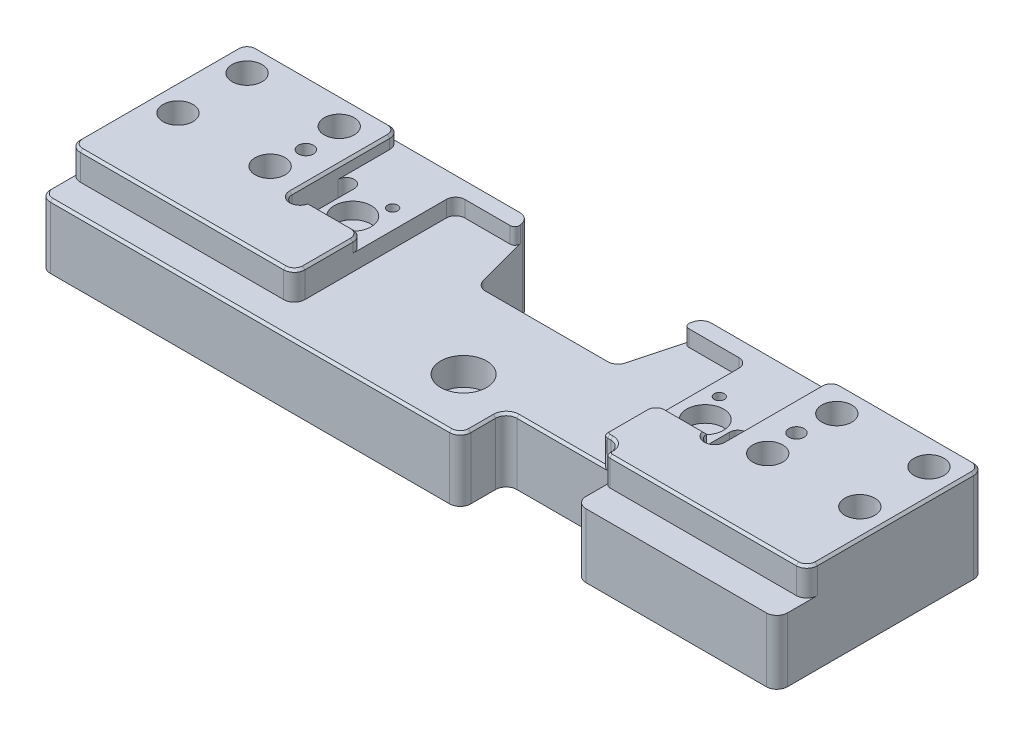
from build123d import *

# Parameters (mm, degrees)
SKETCH1_W                                           = 160
SKETCH1_H                                           = 45
BOSS_EXTRUDE1_DEPTH                                 = 20
SKETCH2_W                                           = 93.5
SKETCH2_H                                           = 23.5
CUT_EXTRUDE1_DEPTH                                  = 2.6
CUT_EXTRUDE14_DEPTH                                 = 3.5
CUT_EXTRUDE7_DEPTH                                  = 86.476604986
SKETCH24_R                                          = 4
SKETCH24_W                                          = 3.5
SKETCH24_H                                          = 10
SKETCH24_H_2                                        = 5
CUT_EXTRUDE16_DEPTH                                 = 3.5
CUT_EXTRUDE17_DEPTH                                 = 10
SKETCH23_R                                          = 1.75
CUT_EXTRUDE15_DEPTH                                 = 10
CUT_EXTRUDE15_DIRECTION_2_REACH                     = 86.906
SKETCH26_R                                          = 1.1
CUT_EXTRUDE18_DEPTH                                 = 12
CBORE_FOR_M3_HEX_SOCKET_HEAD_CAP_SCREW1_D           = 3.4
CBORE_FOR_M3_HEX_SOCKET_HEAD_CAP_SCREW1_CBORE_D     = 6.5
CBORE_FOR_M3_HEX_SOCKET_HEAD_CAP_SCREW1_CBORE_DEPTH = 12.9
SKETCH32_R                                          = 2.525
CUT_EXTRUDE19_DEPTH                                 = 30
M4_TAPPED_HOLE1_D                                   = 3.3
SKETCH35_R                                          = 5
CUT_EXTRUDE20_DEPTH                                 = 6
CUT_EXTRUDE21_DEPTH                                 = 10
CUT_EXTRUDE21_DEPTH_BACK                            = 15
SKETCH36_W                                          = 25
SKETCH36_H                                          = 10
FILLET1_R                                           = 2.3
FILLET2_R                                           = 1
CHAMFER1_SIZE                                       = 0.5


with BuildPart() as part:
    # Sketch1 → Boss-Extrude1 (new body)
    with BuildSketch(Plane(origin=(0, 0, 0), x_dir=(1, 0, 0), z_dir=(0, 1, 0))):
        Rectangle(SKETCH1_W, SKETCH1_H)
    extrude(amount=BOSS_EXTRUDE1_DEPTH)

    # Sketch2 → Cut-Extrude1 (cut)
    with BuildSketch(Plane(origin=(0, 20, 0), x_dir=(1, 0, 0), z_dir=(0, 1, 0))):
        with Locations((0, 10.75)):
            Rectangle(SKETCH2_W, SKETCH2_H)
    extrude(amount=-CUT_EXTRUDE1_DEPTH, mode=Mode.SUBTRACT)

    # Sketch9 → Cut-Extrude14 (cut)
    with BuildSketch(Plane(origin=(0, 17.4, 0), x_dir=(1, 0, 0), z_dir=(0, 1, 0))):
        with BuildLine():
            Line((-29.25, -1), (30.25, -1))
            ThreePointArc((30.25, -1), (31.664213562, -0.414213562), (32.25, 1))
            Line((32.25, 1), (32.25, 17))
            ThreePointArc((32.25, 17), (31.664213562, 18.414213562), (30.25, 19))
            Line((30.25, 19), (-29.25, 19))
            ThreePointArc((-29.25, 19), (-30.664213562, 18.414213562), (-31.25, 17))
            Line((-31.25, 17), (-31.25, 1))
            ThreePointArc((-31.25, 1), (-30.664213562, -0.414213562), (-29.25, -1))
        make_face()
    extrude(amount=-CUT_EXTRUDE14_DEPTH, mode=Mode.SUBTRACT)

    # Sketch12 → Cut-Extrude7 (cut, through all)
    with BuildSketch(Plane(origin=(0, 20, 0), x_dir=(1, 0, 0), z_dir=(0, 1, 0))):
        Polygon((-19.019237886, 22.5), (-15, 7.5), (15, 7.5), (19.019237886, 22.5), align=None)
    extrude(amount=-CUT_EXTRUDE7_DEPTH, mode=Mode.SUBTRACT)

    # Sketch24 → Cut-Extrude16 (cut)
    with BuildSketch(Plane(origin=(0, 17.4, 0), x_dir=(1, 0, 0), z_dir=(0, 1, 0))):
        with Locations(Location((-38.25, 3.675, 0), (0, 0, 270))):
            Circle(SKETCH24_R)
        with Locations(Location((38.25, 3.675, 0), (0, 0, 270))):
            Circle(SKETCH24_R)
        with Locations((-45, 4)):
            Rectangle(SKETCH24_W, SKETCH24_H)
        with Locations((45, 1.5)):
            Rectangle(SKETCH24_W, SKETCH24_H_2)
    extrude(amount=-CUT_EXTRUDE16_DEPTH, mode=Mode.SUBTRACT)

    # Sketch25 → Cut-Extrude17 (cut)
    with BuildSketch(Plane(origin=(0, 13.9, 0), x_dir=(1, 0, 0), z_dir=(0, 1, 0))):
        Polygon((-31.25, 4), (32.25, 4), (32.25, -16), (80, -16), (80, -22.5), (-80, -22.5), (-80, -16), (-31.25, -16), align=None)
    extrude(amount=CUT_EXTRUDE17_DEPTH, mode=Mode.SUBTRACT)

    # Sketch23 → Cut-Extrude15 (cut)
    with BuildSketch(Plane(origin=(0, 17.4, 0), x_dir=(1, 0, 0), z_dir=(0, 1, 0))):
        with Locations((-45, -1)):
            Circle(SKETCH23_R)
        with Locations((45, -1)):
            Circle(SKETCH23_R)
        with Locations((-45, 9)):
            Circle(SKETCH23_R)
        with Locations((45, 4)):
            Circle(SKETCH23_R)
    extrude(amount=CUT_EXTRUDE15_DEPTH, mode=Mode.SUBTRACT)

    # Cut-Extrude15 direction 2: up to this face of the body (flat: up to its plane)
    cut_extrude15_direction_2_end = Plane(part.part.faces().sort_by_distance((-45, 13.9, -4))[0])
    # Sketch23 → Cut-Extrude15 direction 2 (cut, up to the picked face)
    with BuildSketch(Plane(origin=(0, 17.4, 0), x_dir=(1, 0, 0), z_dir=(0, 1, 0)), mode=Mode.PRIVATE) as cut_extrude15_direction_2_sk1:
        with Locations((-45, -1)):
            Circle(SKETCH23_R)
    cut_extrude15_direction_2_tool1 = split(extrude(cut_extrude15_direction_2_sk1.sketch, amount=-CUT_EXTRUDE15_DIRECTION_2_REACH, mode=Mode.PRIVATE), bisect_by=cut_extrude15_direction_2_end, keep=Keep.BOTH, mode=Mode.PRIVATE)
    # Sketch23 → Cut-Extrude15 direction 2 (cut, up to the picked face)
    with BuildSketch(Plane(origin=(0, 17.4, 0), x_dir=(1, 0, 0), z_dir=(0, 1, 0)), mode=Mode.PRIVATE) as cut_extrude15_direction_2_sk2:
        with Locations((45, -1)):
            Circle(SKETCH23_R)
    cut_extrude15_direction_2_tool2 = split(extrude(cut_extrude15_direction_2_sk2.sketch, amount=-CUT_EXTRUDE15_DIRECTION_2_REACH, mode=Mode.PRIVATE), bisect_by=cut_extrude15_direction_2_end, keep=Keep.BOTH, mode=Mode.PRIVATE)
    # Sketch23 → Cut-Extrude15 direction 2 (cut, up to the picked face)
    with BuildSketch(Plane(origin=(0, 17.4, 0), x_dir=(1, 0, 0), z_dir=(0, 1, 0)), mode=Mode.PRIVATE) as cut_extrude15_direction_2_sk3:
        with Locations((-45, 9)):
            Circle(SKETCH23_R)
    cut_extrude15_direction_2_tool3 = split(extrude(cut_extrude15_direction_2_sk3.sketch, amount=-CUT_EXTRUDE15_DIRECTION_2_REACH, mode=Mode.PRIVATE), bisect_by=cut_extrude15_direction_2_end, keep=Keep.BOTH, mode=Mode.PRIVATE)
    # Sketch23 → Cut-Extrude15 direction 2 (cut, up to the picked face)
    with BuildSketch(Plane(origin=(0, 17.4, 0), x_dir=(1, 0, 0), z_dir=(0, 1, 0)), mode=Mode.PRIVATE) as cut_extrude15_direction_2_sk4:
        with Locations((45, 4)):
            Circle(SKETCH23_R)
    cut_extrude15_direction_2_tool4 = split(extrude(cut_extrude15_direction_2_sk4.sketch, amount=-CUT_EXTRUDE15_DIRECTION_2_REACH, mode=Mode.PRIVATE), bisect_by=cut_extrude15_direction_2_end, keep=Keep.BOTH, mode=Mode.PRIVATE)
    add(cut_extrude15_direction_2_tool1.solids().sort_by(Axis((-45, 17.4, 1), (0, -1, 0)))[0], mode=Mode.SUBTRACT)
    add(cut_extrude15_direction_2_tool2.solids().sort_by(Axis((45, 17.4, 1), (0, -1, 0)))[0], mode=Mode.SUBTRACT)
    add(cut_extrude15_direction_2_tool3.solids().sort_by(Axis((-45, 17.4, -9), (0, -1, 0)))[0], mode=Mode.SUBTRACT)
    add(cut_extrude15_direction_2_tool4.solids().sort_by(Axis((45, 17.4, -4), (0, -1, 0)))[0], mode=Mode.SUBTRACT)

    # Sketch26 → Cut-Extrude18 (cut)
    with BuildSketch(Plane(origin=(0, 17.4, 0), x_dir=(1, 0, 0), z_dir=(0, 1, 0))):
        with Locations(Location((35.45, 9.55, 0), (0, 0, 270))):
            Circle(SKETCH26_R)
        with Locations(Location((-35.45, 9.55, 0), (0, 0, 270))):
            Circle(SKETCH26_R)
    extrude(amount=-CUT_EXTRUDE18_DEPTH, mode=Mode.SUBTRACT)

    # CBORE for M3 Hex Socket Head Cap Screw1 (through all)
    with Locations(Plane(origin=(0, 20, 0), x_dir=(1, 0, 0), z_dir=(0, 1, 0))):
        with Locations((-74, 16.5), (-74, 1.5), (-54, 1.5), (-54, 16.5), (54, 16.5), (54, 1.5), (74, 1.5), (74, 16.5)):
            CounterBoreHole(CBORE_FOR_M3_HEX_SOCKET_HEAD_CAP_SCREW1_D / 2, CBORE_FOR_M3_HEX_SOCKET_HEAD_CAP_SCREW1_CBORE_D / 2, CBORE_FOR_M3_HEX_SOCKET_HEAD_CAP_SCREW1_CBORE_DEPTH)

    # Sketch32 → Cut-Extrude19 (cut)
    with BuildSketch(Plane(origin=(0, 13.9, 0), x_dir=(1, 0, 0), z_dir=(0, 1, 0))):
        with Locations(Location((0, -10.5, 0), (0, 0, 270))):
            Circle(SKETCH32_R)
    extrude(amount=-CUT_EXTRUDE19_DEPTH, mode=Mode.SUBTRACT)

    # M4 Tapped Hole1 (through all)
    with Locations(Plane(origin=(0, 20, 0), x_dir=(1, 0, 0), z_dir=(0, 1, 0))):
        with Locations((53.25, 8.5), (-53.25, 8.5)):
            Hole(M4_TAPPED_HOLE1_D / 2)

    # Sketch35 → Cut-Extrude20 (cut)
    with BuildSketch(Plane(origin=(0, 13.9, 0), x_dir=(1, 0, 0), z_dir=(0, 1, 0))):
        with Locations(Location((0, -10.5, 0), (0, 0, 270))):
            Circle(SKETCH35_R)
    extrude(amount=-CUT_EXTRUDE20_DEPTH, mode=Mode.SUBTRACT)

    # Sketch36 → Cut-Extrude21 (cut, two sides: drawn at the far end of the back side and taken through both)
    with BuildSketch(Plane(origin=(0, 13.9, 0), x_dir=(1, 0, 0), z_dir=(0, 1, 0)).offset(-CUT_EXTRUDE21_DEPTH_BACK)):
        with Locations((23.75, -17.5)):
            Rectangle(SKETCH36_W, SKETCH36_H)
    extrude(amount=CUT_EXTRUDE21_DEPTH + CUT_EXTRUDE21_DEPTH_BACK, mode=Mode.SUBTRACT)

    # Fillet1
    fillet1_edges = [part.edges().sort_by_distance(p)[0] for p in [
        (80, 6.95, 22.5),
        (-80, 6.95, 22.5),
        (-31.25, 16.95, 16),
        (-80, 16.95, 16),
        (80, 16.95, 16),
        (-31.25, 18.7, 1),
        (32.25, 18.7, 1),
        (46.75, 18.7, -22.5),
        (-46.75, 18.7, -22.5),
        (36.25, 10, 12.5),
        (36.25, 6.95, 22.5),
        (11.25, 6.95, 12.5),
        (11.25, 6.95, 22.5),
        (-19.019237886, 8.7, -22.5),
        (19.019237886, 8.7, -22.5),
        (15, 6.95, -7.5),
        (-15, 6.95, -7.5),
        (-80, 10, -22.5),
        (80, 10, -22.5),
    ]]
    fillet(fillet1_edges, radius=FILLET1_R)

    # Fillet2
    fillet2_edges = [part.edges().sort_by_distance(p)[0] for p in [
        (36.25, 16.95, 16),
        (32.25, 16.95, 12.5),
        (18.081415713, 15.65, -19),
        (-18.081415713, 15.65, -19),
    ]]
    fillet(fillet2_edges, radius=FILLET2_R)

    # Chamfer1
    chamfer1_edges = [part.edges().sort_by_distance(p)[0] for p in [
        (-80, 13.9, 16.95),
        (-38.4, 20, 1),
        (45, 20, 2.75),
        (-45, 20, 2.75),
        (46.75, 20, -9.6),
        (38.9, 20, 1),
        (57.475, 20, 16),
        (80, 20, -3.25),
        (63.375, 20, -22.5),
        (33.6, 20, 12.5),
        (79.326345597, 20, -21.826345597),
        (79.326345597, 20, 15.326345597),
        (47.423654403, 20, -21.826345597),
        (32.923654403, 20, 1.673654403),
        (-46.75, 20, -9.6),
        (-63.375, 20, -22.5),
        (-80, 20, -3.25),
        (-55.625, 20, 16),
        (-31.25, 20, 8.5),
        (-79.326345597, 20, -21.826345597),
        (-31.923654403, 20, 15.326345597),
        (-79.326345597, 20, 15.326345597),
        (-31.923654403, 20, 1.673654403),
        (-47.423654403, 20, -21.826345597),
        (-34.375, 13.9, 22.5),
        (11.25, 13.9, 17.5),
        (23.4, 13.9, 12.5),
        (10.576345597, 13.9, 21.826345597),
        (-79.326345597, 13.9, 21.826345597),
        (11.923654403, 13.9, 13.173654403),
        (35.576345597, 20, 13.173654403),
        (32.25, 20, 7.4),
        (36.25, 20, 14.9),
        (36.542893219, 20, 15.707106781),
        (32.542893219, 20, 12.207106781),
    ]]
    chamfer(chamfer1_edges, length=CHAMFER1_SIZE)


solid = part.part
